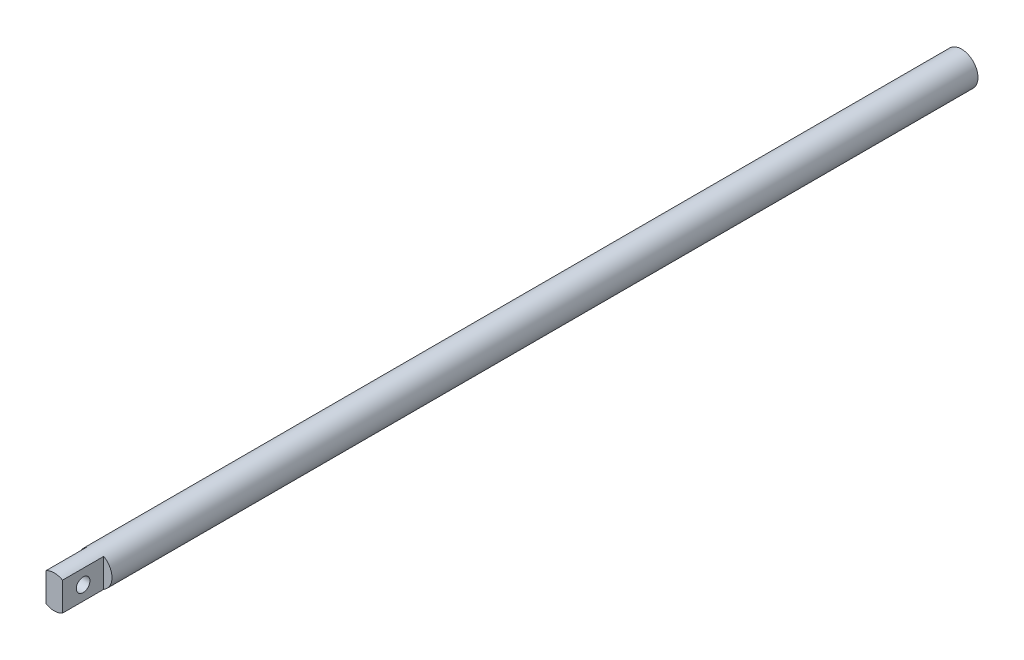
from build123d import *

# Parameters (mm, degrees)
SKETCH1_R               = 20
BOSS_EXTRUDE1_DEPTH     = 1100
CUT_EXTRUDE1_DEPTH      = 1101.363576278
CUT_EXTRUDE1_DEPTH_BACK = 1101.363576278
SKETCH2_W               = 10
SKETCH2_H               = 50
CUT_EXTRUDE2_DEPTH      = 1101.590750461
CUT_EXTRUDE2_DEPTH_BACK = 1101.590750461
SKETCH3_R               = 8.25


with BuildPart() as part:
    # Sketch1 → Boss-Extrude1 (new body)
    with BuildSketch(Plane.XY):
        Circle(SKETCH1_R)
    extrude(amount=BOSS_EXTRUDE1_DEPTH)

    # Sketch2 → Cut-Extrude1 (cut, two sides: drawn at the far end of the back side and taken through both)
    with BuildSketch(Plane(origin=(0, 0, 0), x_dir=(1, 0, 0), z_dir=(0, 1, 0)).offset(-CUT_EXTRUDE1_DEPTH_BACK)):
        with Locations((-15, -1075)):
            Rectangle(SKETCH2_W, SKETCH2_H)
        with Locations((15, -1075)):
            Rectangle(SKETCH2_W, SKETCH2_H)
    extrude(amount=CUT_EXTRUDE1_DEPTH + CUT_EXTRUDE1_DEPTH_BACK, mode=Mode.SUBTRACT)

    # Sketch3 → Cut-Extrude2 (cut, two sides: drawn at the far end of the back side and taken through both)
    with BuildSketch(Plane.ZY.offset(10).offset(-CUT_EXTRUDE2_DEPTH_BACK)):
        with Locations((1075, 0)):
            Circle(SKETCH3_R)
    extrude(amount=CUT_EXTRUDE2_DEPTH + CUT_EXTRUDE2_DEPTH_BACK, mode=Mode.SUBTRACT)


solid = part.part
